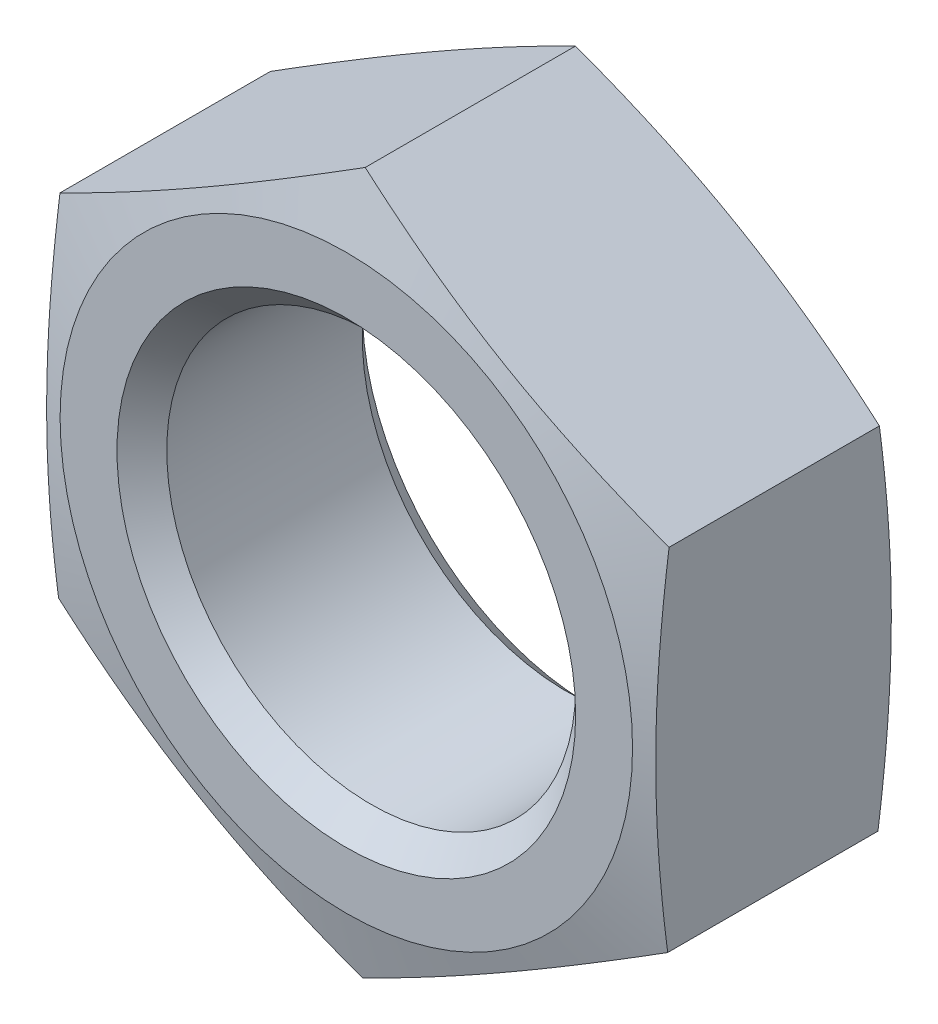
SolidWorks part; units mm, degrees
material "SAE2"
ref_plane "Plane1" through (0, 0, 0) normal (0, 0, 1) x (1, 0, 0)
ref_plane "Plane2" through (0, 0, 0) normal (0, 1, 0) x (1, 0, 0)
ref_plane "Plane3" through (0, 0, 0) normal (1, 0, 0) x (0, 0, -1)
sketch "Dimension sketch" plane through (0, 0, 0) normal (0, 0, 1) x (1, 0, 0)
  line L0 (0, 0) -> (11.5249, 0)
  line L1 (11.5249, 0) -> (37.4249, 0)
  line L2 (37.4249, 0) -> (70.7249, 0)
  line L3 (-22.8571, 0) -> (0, 0)
  point P3 (24, 0)
  point P4 (1.5, 0)
  point P5 (39.55, 0)
  point P6 (21.5, 0)
  point P7 (6.4, 0)
  point P8 (36, 0)
  dimension "D1" = 22.8571
  dimension "D" = 24
  dimension "P" = 1.5
  dimension "e" = 39.55
  dimension "m" = 21.5
  dimension "mw" = 6.4
  dimension "s" = 36
  dimension "da" = 25.9
  dimension "dw" = 33.3
sketch "Sketch1" plane through (0, 0, 0) normal (0, 0, 1) x (1, 0, 0)
  line L0 (-26.8088, 0) -> (37.1748, 0) construction
  line L1 (0, 25.0215) -> (0, -25.0215) construction
  line L3 (0.0846, 21.4998) -> (-18.5771, 10.8232)
  line L4 (-18.5771, 10.8232) -> (-18.6617, -10.6767)
  line L5 (-18.6617, -10.6767) -> (-0.0846, -21.4998)
  line L6 (-0.0846, -21.4998) -> (18.5771, -10.8232)
  line L7 (18.5771, -10.8232) -> (18.6617, 10.6767)
  line L8 (18.6617, 10.6767) -> (0.0846, 21.4998)
  circle A0 centre (0, 0) radius 18.6195 construction
  circle A1 centre (0, 0) radius 12.5
  dimension "D" = 25
  dimension "e" = 43
extrude "Base-Extrude" add sketch "Sketch1" along normal blind 15
sketch "Sketch2" plane through (0, 0, 0) normal (0, 0, -1) x (-1, 0, 0)
  circle A0 centre (0, 0) radius 17.5
  circle A1 centre (0, 0) radius 12.5 construction
  dimension "s" = 35
extrude "Cut-Extrude1" cut sketch "Sketch2" against normal through all draft 75 flip side to cut
sketch "Sketch3" plane through (0, 0, 15) normal (0, 0, 1) x (1, 0, 0)
  circle A0 centre (0, 0) radius 17.5
  dimension "D1" = 35
extrude "Cut-Extrude2" cut sketch "Sketch3" against normal through all draft 75 flip side to cut
chamfer "Chamfer1" distance 1.5214 angle 45 2 edges at (12.5, 0, 0) (12.5, 0, 15)
